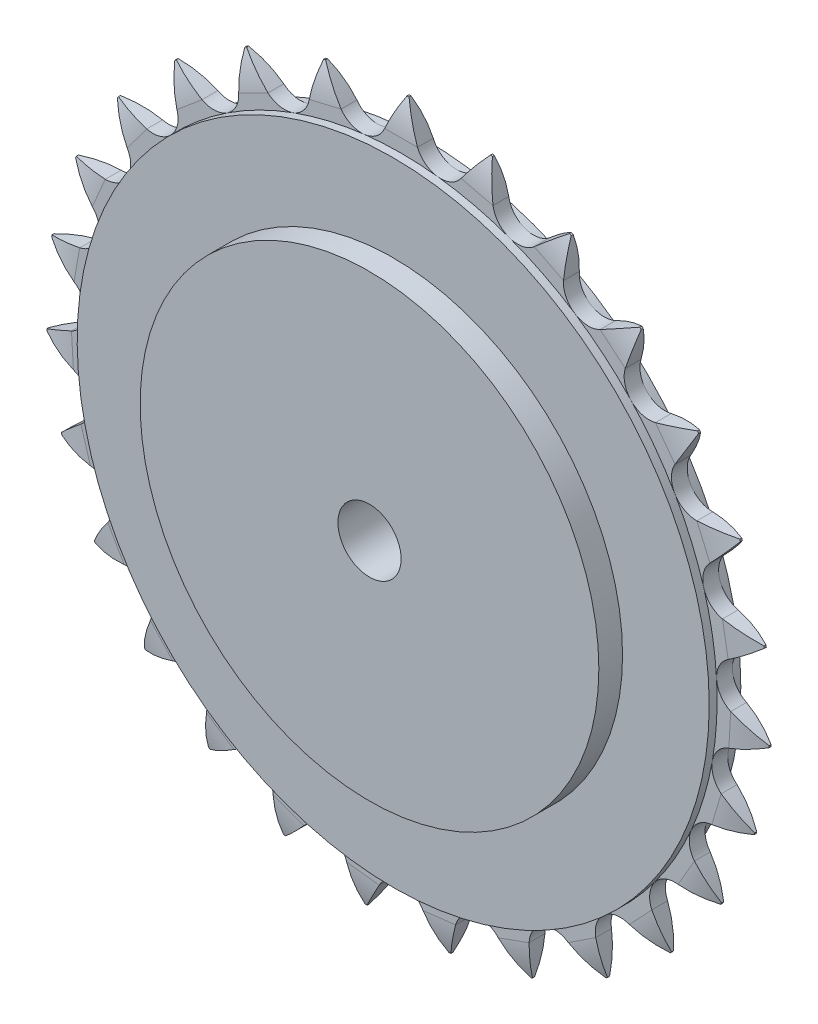
from build123d import *

# Parameters (mm, degrees)
BOSS_EXTRUDE1_DEPTH      = 2
BOSS_EXTRUDE1_DEPTH_BACK = 2
CUT_EXTRUDE1_DEPTH       = 12
CUT_EXTRUDE1_DEPTH_BACK  = 12
CIRPATTERN1_COUNT        = 27
SKETCH8_R                = 80.003940092
BOSS_EXTRUDE4_DEPTH      = 4
SKETCH9_R                = 58.064259058
BOSS_EXTRUDE5_DEPTH      = 10
SCALE6_SCALE             = 0.5
SCALE7_SCALE             = 0.5
SCALE8_SCALE             = 0.5
SKETCH10_R               = 1
CUT_EXTRUDE3_DEPTH       = 17.266878635


with BuildPart() as part:
    # Sketch3 → Boss-Extrude1 (new, two sides: drawn at the far end of the back side and taken through both)
    with BuildSketch(Plane.XY.offset(-BOSS_EXTRUDE1_DEPTH_BACK)):
        with BuildLine():
            Line((-0.25, 91.55546781), (0.25, 91.55546781))
            ThreePointArc((0.25, 91.55546781), (2.304999029, 87.501396725), (4.15, 83.347544923))
            ThreePointArc((4.15, 83.347544923), (6.190786455, 80.70669784), (9.287890547, 79.46298207))
            ThreePointArc((9.287890547, 79.46298207), (0, 80.003940092), (-9.287890547, 79.46298207))
            ThreePointArc((-9.287890547, 79.46298207), (-6.190786455, 80.70669784), (-4.15, 83.347544923))
            ThreePointArc((-4.15, 83.347544923), (-2.304999029, 87.501396725), (-0.25, 91.55546781))
        make_face()
    extrude(amount=BOSS_EXTRUDE1_DEPTH + BOSS_EXTRUDE1_DEPTH_BACK)

    # Sketch4 → Cut-Extrude1 (cut, two sides: drawn at the far end of the back side and taken through both)
    with BuildSketch(Plane(origin=(0, 0, 0), x_dir=(0, 0, -1), z_dir=(1, 0, 0)).offset(-CUT_EXTRUDE1_DEPTH_BACK)):
        with BuildLine():
            Line((-0.25, 91.55546781), (0.25, 91.55546781))
            ThreePointArc((0.25, 91.55546781), (1.471881784, 87.525464557), (2, 83.347544923))
            Line((2, 83.347544923), (4.331469649, 83.347544923))
            Line((4.331469649, 83.347544923), (4.331469649, 94.150918421))
            Line((4.331469649, 94.150918421), (-4.867818658, 94.150918421))
            Line((-4.867818658, 94.150918421), (-4.867818658, 83.347544923))
            Line((-4.867818658, 83.347544923), (-2, 83.347544923))
            ThreePointArc((-2, 83.347544923), (-1.471881784, 87.525464557), (-0.25, 91.55546781))
        make_face()
    extrude(amount=CUT_EXTRUDE1_DEPTH + CUT_EXTRUDE1_DEPTH_BACK, mode=Mode.SUBTRACT)


with BuildPart() as cirpattern1_1:
    # CirPattern1: pattern copy
    add(part.part.rotate(Axis((0, 0, 0), (0, 0, 1)), 1 * 360 / CIRPATTERN1_COUNT))


with BuildPart() as cirpattern1_2:
    # CirPattern1: pattern copy
    add(part.part.rotate(Axis((0, 0, 0), (0, 0, 1)), 2 * 360 / CIRPATTERN1_COUNT))


with BuildPart() as cirpattern1_3:
    # CirPattern1: pattern copy
    add(part.part.rotate(Axis((0, 0, 0), (0, 0, 1)), 3 * 360 / CIRPATTERN1_COUNT))


with BuildPart() as cirpattern1_4:
    # CirPattern1: pattern copy
    add(part.part.rotate(Axis((0, 0, 0), (0, 0, 1)), 4 * 360 / CIRPATTERN1_COUNT))


with BuildPart() as cirpattern1_5:
    # CirPattern1: pattern copy
    add(part.part.rotate(Axis((0, 0, 0), (0, 0, 1)), 5 * 360 / CIRPATTERN1_COUNT))


with BuildPart() as cirpattern1_6:
    # CirPattern1: pattern copy
    add(part.part.rotate(Axis((0, 0, 0), (0, 0, 1)), 6 * 360 / CIRPATTERN1_COUNT))


with BuildPart() as cirpattern1_7:
    # CirPattern1: pattern copy
    add(part.part.rotate(Axis((0, 0, 0), (0, 0, 1)), 7 * 360 / CIRPATTERN1_COUNT))


with BuildPart() as cirpattern1_8:
    # CirPattern1: pattern copy
    add(part.part.rotate(Axis((0, 0, 0), (0, 0, 1)), 8 * 360 / CIRPATTERN1_COUNT))


with BuildPart() as cirpattern1_9:
    # CirPattern1: pattern copy
    add(part.part.rotate(Axis((0, 0, 0), (0, 0, 1)), 9 * 360 / CIRPATTERN1_COUNT))


with BuildPart() as cirpattern1_10:
    # CirPattern1: pattern copy
    add(part.part.rotate(Axis((0, 0, 0), (0, 0, 1)), 10 * 360 / CIRPATTERN1_COUNT))


with BuildPart() as cirpattern1_11:
    # CirPattern1: pattern copy
    add(part.part.rotate(Axis((0, 0, 0), (0, 0, 1)), 11 * 360 / CIRPATTERN1_COUNT))


with BuildPart() as cirpattern1_12:
    # CirPattern1: pattern copy
    add(part.part.rotate(Axis((0, 0, 0), (0, 0, 1)), 12 * 360 / CIRPATTERN1_COUNT))


with BuildPart() as cirpattern1_13:
    # CirPattern1: pattern copy
    add(part.part.rotate(Axis((0, 0, 0), (0, 0, 1)), 13 * 360 / CIRPATTERN1_COUNT))


with BuildPart() as cirpattern1_14:
    # CirPattern1: pattern copy
    add(part.part.rotate(Axis((0, 0, 0), (0, 0, 1)), 14 * 360 / CIRPATTERN1_COUNT))


with BuildPart() as cirpattern1_15:
    # CirPattern1: pattern copy
    add(part.part.rotate(Axis((0, 0, 0), (0, 0, 1)), 15 * 360 / CIRPATTERN1_COUNT))


with BuildPart() as cirpattern1_16:
    # CirPattern1: pattern copy
    add(part.part.rotate(Axis((0, 0, 0), (0, 0, 1)), 16 * 360 / CIRPATTERN1_COUNT))


with BuildPart() as cirpattern1_17:
    # CirPattern1: pattern copy
    add(part.part.rotate(Axis((0, 0, 0), (0, 0, 1)), 17 * 360 / CIRPATTERN1_COUNT))


with BuildPart() as cirpattern1_18:
    # CirPattern1: pattern copy
    add(part.part.rotate(Axis((0, 0, 0), (0, 0, 1)), 18 * 360 / CIRPATTERN1_COUNT))


with BuildPart() as cirpattern1_19:
    # CirPattern1: pattern copy
    add(part.part.rotate(Axis((0, 0, 0), (0, 0, 1)), 19 * 360 / CIRPATTERN1_COUNT))


with BuildPart() as cirpattern1_20:
    # CirPattern1: pattern copy
    add(part.part.rotate(Axis((0, 0, 0), (0, 0, 1)), 20 * 360 / CIRPATTERN1_COUNT))


with BuildPart() as cirpattern1_21:
    # CirPattern1: pattern copy
    add(part.part.rotate(Axis((0, 0, 0), (0, 0, 1)), 21 * 360 / CIRPATTERN1_COUNT))


with BuildPart() as cirpattern1_22:
    # CirPattern1: pattern copy
    add(part.part.rotate(Axis((0, 0, 0), (0, 0, 1)), 22 * 360 / CIRPATTERN1_COUNT))


with BuildPart() as cirpattern1_23:
    # CirPattern1: pattern copy
    add(part.part.rotate(Axis((0, 0, 0), (0, 0, 1)), 23 * 360 / CIRPATTERN1_COUNT))


with BuildPart() as cirpattern1_24:
    # CirPattern1: pattern copy
    add(part.part.rotate(Axis((0, 0, 0), (0, 0, 1)), 24 * 360 / CIRPATTERN1_COUNT))


with BuildPart() as cirpattern1_25:
    # CirPattern1: pattern copy
    add(part.part.rotate(Axis((0, 0, 0), (0, 0, 1)), 25 * 360 / CIRPATTERN1_COUNT))


with BuildPart() as cirpattern1_26:
    # CirPattern1: pattern copy
    add(part.part.rotate(Axis((0, 0, 0), (0, 0, 1)), 26 * 360 / CIRPATTERN1_COUNT))


with BuildPart() as part_1:
    add(part.part)

    add(cirpattern1_1.part)  # Boss-Extrude4 merges CirPattern1_1

    add(cirpattern1_2.part)  # Boss-Extrude4 merges CirPattern1_2

    add(cirpattern1_3.part)  # Boss-Extrude4 merges CirPattern1_3

    add(cirpattern1_4.part)  # Boss-Extrude4 merges CirPattern1_4

    add(cirpattern1_5.part)  # Boss-Extrude4 merges CirPattern1_5

    add(cirpattern1_6.part)  # Boss-Extrude4 merges CirPattern1_6

    add(cirpattern1_7.part)  # Boss-Extrude4 merges CirPattern1_7

    add(cirpattern1_8.part)  # Boss-Extrude4 merges CirPattern1_8

    add(cirpattern1_9.part)  # Boss-Extrude4 merges CirPattern1_9

    add(cirpattern1_10.part)  # Boss-Extrude4 merges CirPattern1_10

    add(cirpattern1_11.part)  # Boss-Extrude4 merges CirPattern1_11

    add(cirpattern1_12.part)  # Boss-Extrude4 merges CirPattern1_12

    add(cirpattern1_13.part)  # Boss-Extrude4 merges CirPattern1_13

    add(cirpattern1_14.part)  # Boss-Extrude4 merges CirPattern1_14

    add(cirpattern1_15.part)  # Boss-Extrude4 merges CirPattern1_15

    add(cirpattern1_16.part)  # Boss-Extrude4 merges CirPattern1_16

    add(cirpattern1_17.part)  # Boss-Extrude4 merges CirPattern1_17

    add(cirpattern1_18.part)  # Boss-Extrude4 merges CirPattern1_18

    add(cirpattern1_19.part)  # Boss-Extrude4 merges CirPattern1_19

    add(cirpattern1_20.part)  # Boss-Extrude4 merges CirPattern1_20

    add(cirpattern1_21.part)  # Boss-Extrude4 merges CirPattern1_21

    add(cirpattern1_22.part)  # Boss-Extrude4 merges CirPattern1_22

    add(cirpattern1_23.part)  # Boss-Extrude4 merges CirPattern1_23

    add(cirpattern1_24.part)  # Boss-Extrude4 merges CirPattern1_24

    add(cirpattern1_25.part)  # Boss-Extrude4 merges CirPattern1_25

    add(cirpattern1_26.part)  # Boss-Extrude4 merges CirPattern1_26
    # Sketch8 → Boss-Extrude4 (add, symmetric)
    with BuildSketch(Plane.XY):
        with Locations(Location((0, 0, 0), (0, 0, 176.666666667))):
            Circle(SKETCH8_R)
    extrude(amount=BOSS_EXTRUDE4_DEPTH, both=True)

    # Sketch9 → Boss-Extrude5 (add)
    with BuildSketch(Plane.XY):
        Circle(SKETCH9_R)
    extrude(amount=BOSS_EXTRUDE5_DEPTH)


with BuildPart() as part_2:
    # Scale6: scaled about (0, 0, 1.919291741)
    add(part_1.part.scale(SCALE6_SCALE).moved(Location((0, 0, 0.959645871))))


with BuildPart() as part_3:
    # Scale7: scaled about (0, 0, 1.919291741)
    add(part_2.part.scale(SCALE7_SCALE).moved(Location((0, 0, 0.959645871))))


with BuildPart() as part_4:
    # Scale8: scaled about (0, 0, 1.919291741)
    add(part_3.part.scale(SCALE8_SCALE).moved(Location((0, 0, 0.959645871))))

    # Sketch10 → Cut-Extrude3 (cut, through all)
    with BuildSketch(Plane.XY.offset(2.929380671)):
        with Locations((0, -0.120907857)):
            Circle(SKETCH10_R)
    extrude(amount=-CUT_EXTRUDE3_DEPTH, mode=Mode.SUBTRACT)


solid = part_4.part
